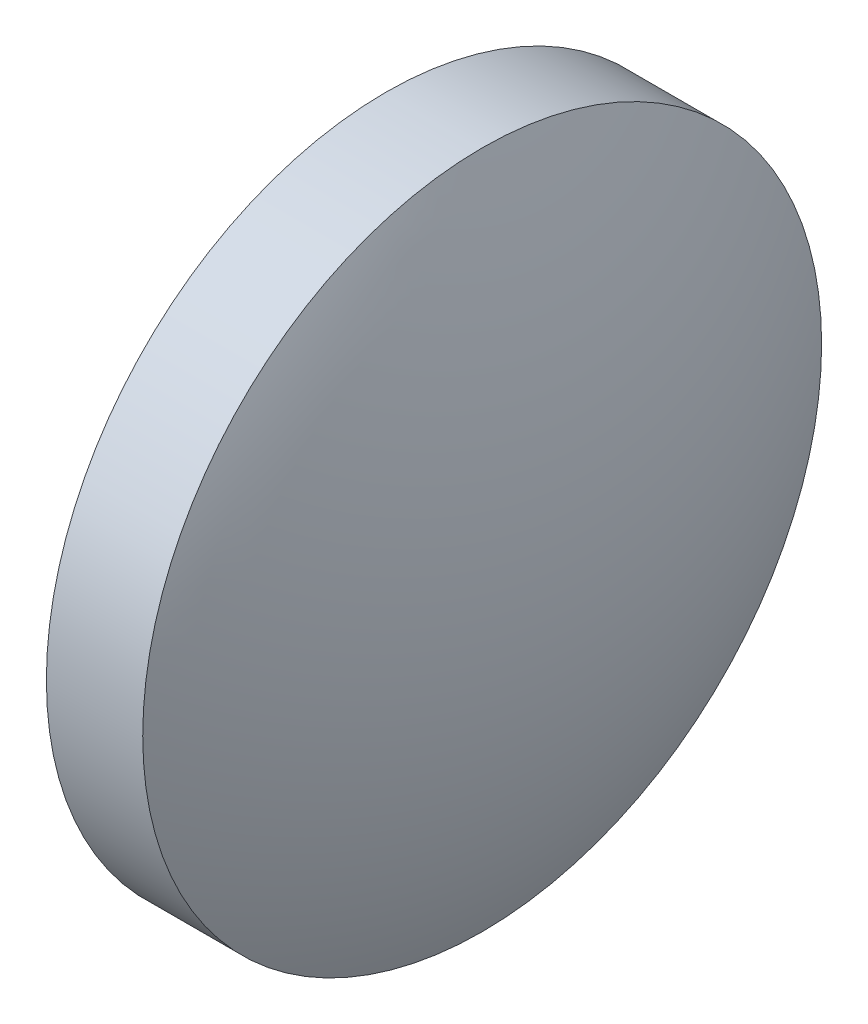
SolidWorks part; units mm, degrees
ref_plane "Front Plane" through (0, 0, 0) normal (0, 0, 1) x (1, 0, 0)
ref_plane "Top Plane" through (0, 0, 0) normal (0, 1, 0) x (1, 0, 0)
ref_plane "Right Plane" through (0, 0, 0) normal (1, 0, 0) x (0, 0, -1)
sketch "Sketch1" plane through (0, 0, 0) normal (0, 0, 1) x (1, 0, 0)
  line L0 (14.64, 0) -> (9.94, 0)
  line L1 (11.3888, 6.35) -> (13.1912, 6.35)
  line L2 (14.64, 0) -> (9.94, 0) construction
  arc A4 (14.64, 0) -> (13.1912, 6.35) centre (0, 0) ccw
  arc A5 (11.3888, 6.35) -> (9.94, 0) centre (24.58, 0) ccw
revolve "Revolve4" add sketch "Sketch1" angle 360 about L2
